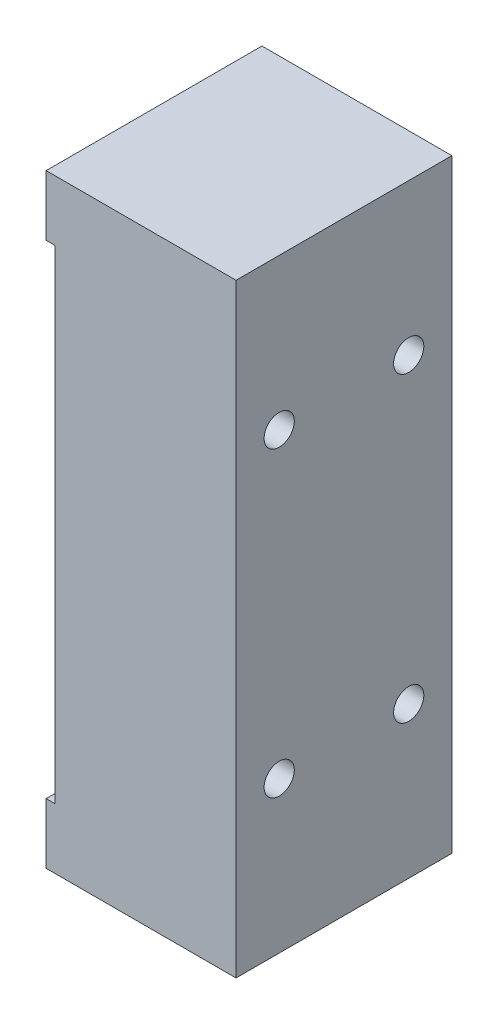
from build123d import *

# Parameters (mm, degrees)
SKETCH1_W           = 22
SKETCH1_H           = 25
BOSS_EXTRUDE1_DEPTH = 70
SKETCH2_R           = 1.75
CUT_EXTRUDE1_DEPTH  = 75.432855649
SKETCH4_W           = 25
SKETCH4_H           = 56
CUT_EXTRUDE3_DEPTH  = 1


with BuildPart() as part:
    # Sketch1 → Boss-Extrude1 (new body)
    with BuildSketch(Plane(origin=(0, 0, 0), x_dir=(1, 0, 0), z_dir=(0, 1, 0))):
        Rectangle(SKETCH1_W, SKETCH1_H)
    extrude(amount=BOSS_EXTRUDE1_DEPTH)

    # Sketch2 → Cut-Extrude1 (cut, through all)
    with BuildSketch(Plane(origin=(11, 0, 0), x_dir=(0, 0, -1), z_dir=(1, 0, 0))):
        with Locations((-7.5, 52.5)):
            Circle(SKETCH2_R)
        with Locations(Location((7.5, 52.5, 0), (0, 0, 180))):
            Circle(SKETCH2_R)
        with Locations((7.5, 17.5)):
            Circle(SKETCH2_R)
        with Locations(Location((-7.5, 17.5, 0), (0, 0, 180))):
            Circle(SKETCH2_R)
    extrude(amount=-CUT_EXTRUDE1_DEPTH, mode=Mode.SUBTRACT)

    # Sketch4 → Cut-Extrude3 (cut)
    with BuildSketch(Plane.ZY.offset(11)):
        with Locations((0, 35)):
            Rectangle(SKETCH4_W, SKETCH4_H)
    extrude(amount=-CUT_EXTRUDE3_DEPTH, mode=Mode.SUBTRACT)


solid = part.part
